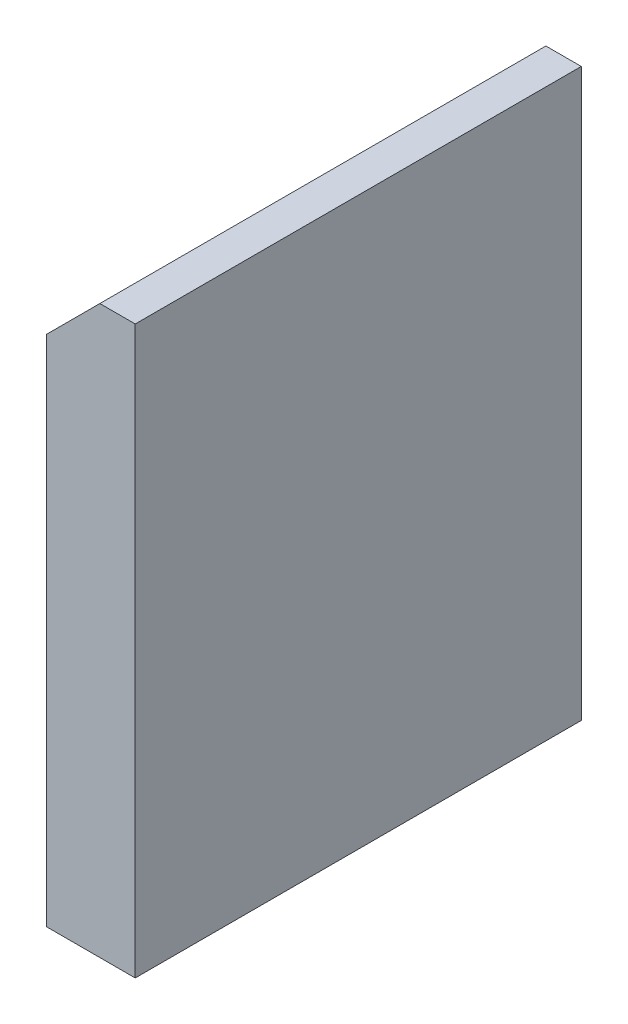
SolidWorks part; units mm, degrees
material "Q345B"
ref_plane "Front Plane" through (0, 0, 0) normal (0, 0, 1) x (1, 0, 0)
ref_plane "Top Plane" through (0, 0, 0) normal (0, 1, 0) x (1, 0, 0)
ref_plane "Right Plane" through (0, 0, 0) normal (1, 0, 0) x (0, 0, -1)
sketch "Sketch2" plane through (0, 0, 0) normal (0, 1, 0) x (1, 0, 0)
  line L0 (-131.395, 0) -> (113.7022, 0) construction
  line L1 (0, 164.1787) -> (0, -121.5078) construction
  line L3 (-12.5, 63) -> (12.5, 63)
  line L4 (-12.5, 63) -> (-12.5, -63)
  line L5 (-12.5, -63) -> (12.5, -63)
  line L6 (12.5, 63) -> (12.5, -63)
  dimension "D1" = 126
  dimension "D2" = 25
  dimension "D3" = 12.5
extrude "Boss-Extrude1" add sketch "Sketch2" along normal mid plane 160
chamfer "Chamfer1" distance 15 angle 45 1 edges at (-12.5, 80, 0)
